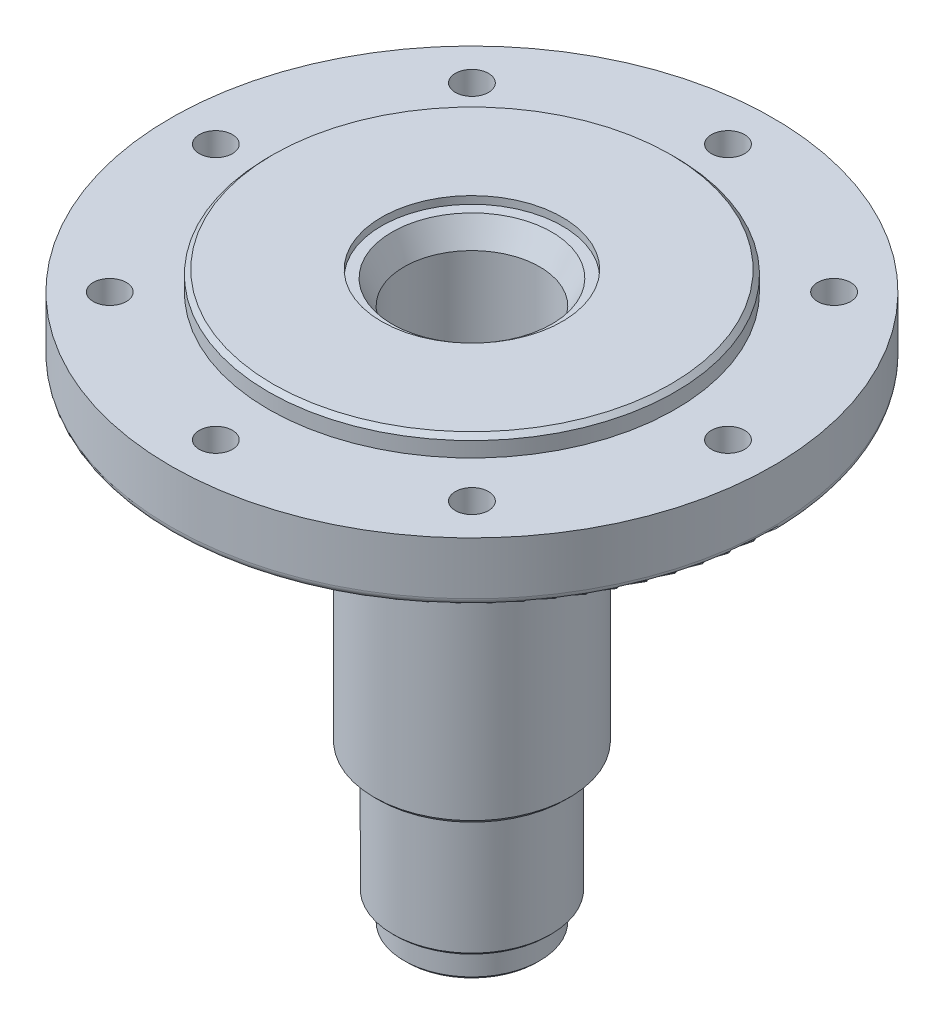
SolidWorks part; units mm, degrees
ref_plane "前视基准面" through (0, 0, 0) normal (0, 0, 1) x (1, 0, 0)
ref_plane "上视基准面" through (0, 0, 0) normal (0, 1, 0) x (1, 0, 0)
ref_plane "右视基准面" through (0, 0, 0) normal (1, 0, 0) x (0, 0, -1)
sketch "草图1" plane through (0, 0, 0) normal (0, 0, 1) x (1, 0, 0)
  line L0 (0, 246.1424) -> (0, -261.2431) construction
  line L1 (60, 198.0206) -> (132, 198.0206)
  line L2 (60, 198.0206) -> (60, 193.0206)
  line L3 (135, 195.0206) -> (135, 185.0206)
  line L4 (135, 185.0206) -> (200, 185.0206)
  line L5 (200, 185.0206) -> (200, 150.0206)
  line L6 (195, 145.0206) -> (145, 145.0206)
  line L7 (145, 145.0206) -> (145, 140.0206)
  line L8 (145, 140.0206) -> (80, 140.0206)
  line L9 (80, 140.0206) -> (80, 87.0206)
  line L10 (77, 84.0206) -> (65, 84.0206)
  line L11 (65, 84.0206) -> (65, -72.9794)
  line L12 (62, -75.9794) -> (52.5, -75.9794)
  line L13 (52.5, -75.9794) -> (52.5, -131.9794)
  line L14 (50.5, -133.9794) -> (45, -133.9794)
  line L15 (45, -133.9794) -> (45, -167.9794)
  line L16 (44, -168.9794) -> (30, -168.9794)
  line L17 (30, -168.9794) -> (30, -36.9794)
  line L18 (30, -36.9794) -> (45, -20.4794)
  line L19 (45, -20.4794) -> (45, 177.0206)
  line L20 (60, 193.0206) -> (53, 193.0206)
  line L21 (53, 193.0206) -> (45, 177.0206)
  line L23 (50.5, -133.9794) -> (52.5, -133.9794)
  line L24 (65, -72.9794) -> (62, -75.9794)
  line L25 (80, 87.0206) -> (77, 84.0206)
  line L26 (132, 198.0206) -> (135, 195.0206)
  line L27 (52.5, -133.9794) -> (52.5, -131.9794)
  line L28 (45, -167.9794) -> (45, -168.9794)
  line L29 (45, -168.9794) -> (44, -168.9794)
  arc A0 (195, 145.0206) -> (200, 150.0206) centre (195, 150.0206) ccw
  point P4 (135, 198.0206)
  point P5 (45, -168.9794)
  point P13 (80, 84.0206)
  point P15 (65, -75.9794)
  point P17 (52.5, -133.9794)
  point P34 (200, 145.0206)
  dimension "D23" = 5
  dimension "D1" = 60
  dimension "D2" = 75
  dimension "D3" = 13
  dimension "D4" = 65
  dimension "D5" = 40
  dimension "D6" = 55
  dimension "D7" = 5
  dimension "D8" = 65
  dimension "D9" = 56
  dimension "D10" = 15
  dimension "D11" = 160
  dimension "D12" = 12.5
  dimension "D13" = 58
  dimension "D14" = 7.5
  dimension "D15" = 35
  dimension "D16" = 15
  dimension "D17" = 132
  dimension "D18" = 90
  dimension "D19" = 197.5
  dimension "D20" = 5
  dimension "D21" = 7
  dimension "D22" = 16
revolve "旋转1" add sketch "草图1" angle 360 about L0
sketch "草图2" plane through (0, 145.0206, 0) normal (0, -1, 0) x (1, 0, 0)
  circle A0 centre (-120.2082, 120.2082) radius 20
  circle A1 centre (-170, 0) radius 20
  circle A2 centre (0, 170) radius 20
  circle A3 centre (120.2082, 120.2082) radius 20
  circle A4 centre (170, 0) radius 20
  circle A5 centre (120.2082, -120.2082) radius 20
  circle A6 centre (0, -170) radius 20
  circle A7 centre (-120.2082, -120.2082) radius 20
  point P19 (0, 0)
  dimension "D1" = 8
  dimension "D2" = 40
extrude "切除-拉伸1" cut sketch "草图2" against normal blind 5
sketch "草图3" plane through (0, 145.0206, 0) normal (0, -1, 0) x (1, 0, 0)
  circle A0 centre (-170, 0) radius 11
  circle A1 centre (-120.2082, 120.2082) radius 11
  circle A2 centre (0, 170) radius 11
  circle A3 centre (120.2082, 120.2082) radius 11
  circle A4 centre (170, 0) radius 11
  circle A5 centre (120.2082, -120.2082) radius 11
  circle A6 centre (0, -170) radius 11
  circle A7 centre (-120.2082, -120.2082) radius 11
  point P19 (0, 0)
  dimension "D1" = 22
  dimension "D2" = 8
extrude "切除-拉伸2" cut sketch "草图3" against normal up to next
sketch "草图5" plane through (0, 140.0206, 0) normal (0, -1, 0) x (1, 0, 0)
  circle A0 centre (0, 0) radius 120
  circle A2 centre (0, 0) radius 80
  circle A3 centre (0, 0) radius 80
  dimension "D1" = 240
  dimension "D2" = 0
extrude "切除-拉伸3" cut sketch "草图5" against normal blind 8
sketch "草图6" plane through (0, -133.9794, 0) normal (0, -1, 0) x (1, 0, 0)
  circle A0 centre (0, 0) radius 52.5 construction
  circle A1 centre (0, 0) radius 45
  circle A2 centre (0, 0) radius 45
  circle A3 centre (0, 0) radius 52.5
  dimension "D1" = 0
extrude "凸台-拉伸1" add sketch "草图6" along normal blind 26
sketch "草图7" plane through (0, -168.9794, 0) normal (0, -1, 0) x (1, 0, 0)
  circle A0 centre (0, 0) radius 45 construction
  circle A1 centre (0, 0) radius 30
  circle A2 centre (0, 0) radius 30
  circle A3 centre (0, 0) radius 45
  dimension "D1" = 0
extrude "凸台-拉伸2" add sketch "草图7" along normal blind 10
chamfer "倒角1" distance 2 angle 45 1 edges at (0, -159.9794, -52.5)
chamfer "倒角2" distance 2 angle 45 1 edges at (0, -178.9794, -45)
